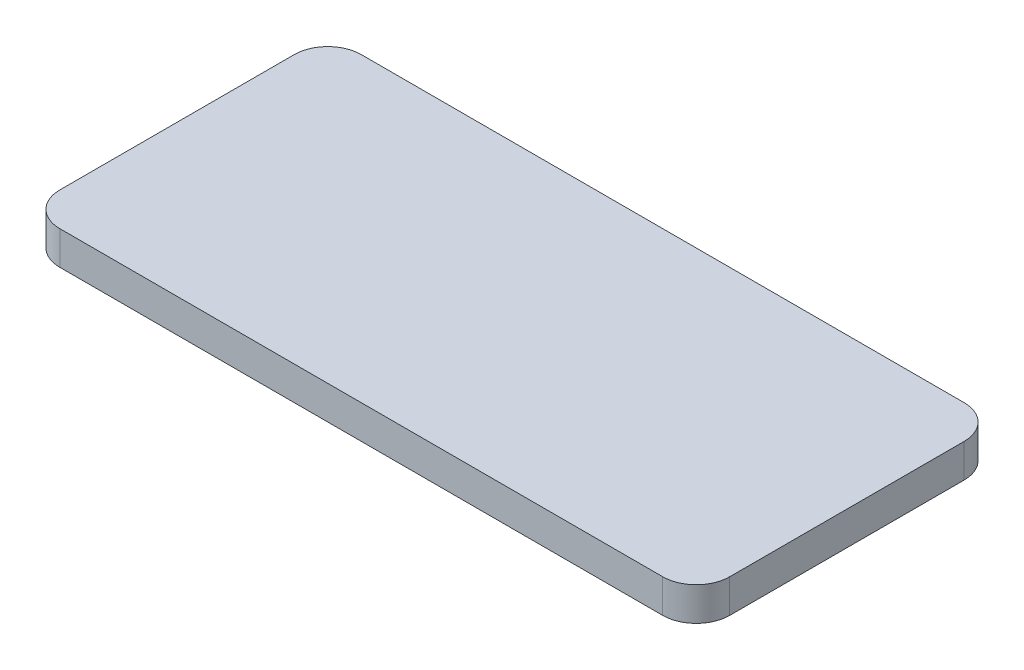
from build123d import *

# Parameters (mm, degrees)
SKETCH1_W           = 200
SKETCH1_H           = 90
BOSS_EXTRUDE1_DEPTH = 10
FILLET1_R           = 10


with BuildPart() as part:
    # Sketch1 → Boss-Extrude1 (new body)
    with BuildSketch(Plane(origin=(0, 0, 0), x_dir=(1, 0, 0), z_dir=(0, 1, 0))):
        with Locations((100, 45)):
            Rectangle(SKETCH1_W, SKETCH1_H)
    extrude(amount=BOSS_EXTRUDE1_DEPTH)

    # Fillet1
    fillet1_edges = [part.edges().sort_by_distance(p)[0] for p in [
        (0, 5, -90),
        (200, 5, -90),
        (200, 5, 0),
        (0, 5, 0),
    ]]
    fillet(fillet1_edges, radius=FILLET1_R)


solid = part.part
